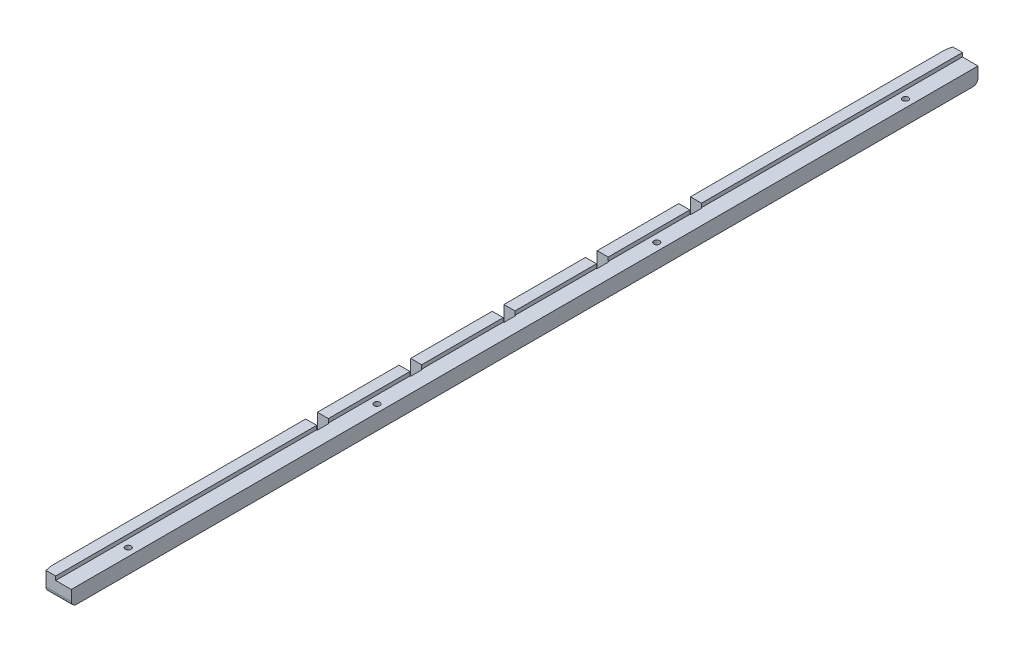
from build123d import *

# Parameters (mm, degrees)
EXTRUDE_1_DEPTH           = 700
HOLE_WIZARD_1_D           = 4.5
HOLE_WIZARD_1_CBORE_D     = 8
HOLE_WIZARD_1_CBORE_DEPTH = 4.6
SKETCH_5_W                = 9
SKETCH_5_H                = 15
CUT_EXTRUDE_1_DEPTH       = 9
CHAMFER_1_SIZE            = 5
CHAMFER_1_SIZE2           = 1
CHAMFER_2_SIZE            = 1
CHAMFER_2_SIZE2           = 5
FILLET_1_R                = 4


with BuildPart() as part:
    # 草图1 → 凸台-拉伸1 (new body)
    with BuildSketch(Plane.XY):
        Polygon((-9.367113838, -5.483188588), (11.132886162, -5.483188588), (11.132886162, 6.516811412), (-0.867113838, 6.516811412), (-0.867113838, 9.516811412), (-9.367113838, 9.516811412), align=None)
    extrude(amount=EXTRUDE_1_DEPTH)

    # 打孔尺寸根据内六角圆柱头螺钉的类型1 (through all)
    with Locations(Plane(origin=(0, -5.483188588, 0), x_dir=(-1, 0, 0), z_dir=(0, -1, 0))):
        with Locations((-5.132886162, -650), (-5.132886162, -458), (-5.132886162, -242), (-5.132886162, -50)):
            CounterBoreHole(HOLE_WIZARD_1_D / 2, HOLE_WIZARD_1_CBORE_D / 2, HOLE_WIZARD_1_CBORE_DEPTH)

    # 草图5 → 切除-拉伸1 (cut)
    with BuildSketch(Plane.ZY.offset(9.367113838)):
        with Locations((206, 2.016811412)):
            Rectangle(SKETCH_5_W, SKETCH_5_H)
        with Locations((278, 2.016811412)):
            Rectangle(SKETCH_5_W, SKETCH_5_H)
        with Locations((350, 2.016811412)):
            Rectangle(SKETCH_5_W, SKETCH_5_H)
        with Locations((422, 2.016811412)):
            Rectangle(SKETCH_5_W, SKETCH_5_H)
        with Locations((494, 2.016811412)):
            Rectangle(SKETCH_5_W, SKETCH_5_H)
    extrude(amount=-CUT_EXTRUDE_1_DEPTH, mode=Mode.SUBTRACT)

    # 倒角1
    chamfer_1_edges = [part.edges().sort_by_distance(p)[0] for p in [
        (-9.367113838, 2.016811412, 700),
    ]]
    chamfer_1_side = [part.faces().sort_by_distance(p)[0] for p in [
        (-9.367113838, 2.016811412, 599.25),
    ]]
    chamfer(chamfer_1_edges, length=CHAMFER_1_SIZE, length2=CHAMFER_1_SIZE2, reference=chamfer_1_side[0])

    # 倒角2
    chamfer_2_edges = [part.edges().sort_by_distance(p)[0] for p in [
        (-9.367113838, 2.016811412, 0),
    ]]
    chamfer_2_side = [part.faces().sort_by_distance(p)[0] for p in [
        (0.31935025, 1.221231301, 0),
    ]]
    chamfer(chamfer_2_edges, length=CHAMFER_2_SIZE, length2=CHAMFER_2_SIZE2, reference=chamfer_2_side[0])

    # 圆角1
    fillet_1_edges = [part.edges().sort_by_distance(p)[0] for p in [
        (1.382886162, -5.483188588, 700),
        (1.382886162, -5.483188588, 0),
    ]]
    fillet(fillet_1_edges, radius=FILLET_1_R)


solid = part.part
